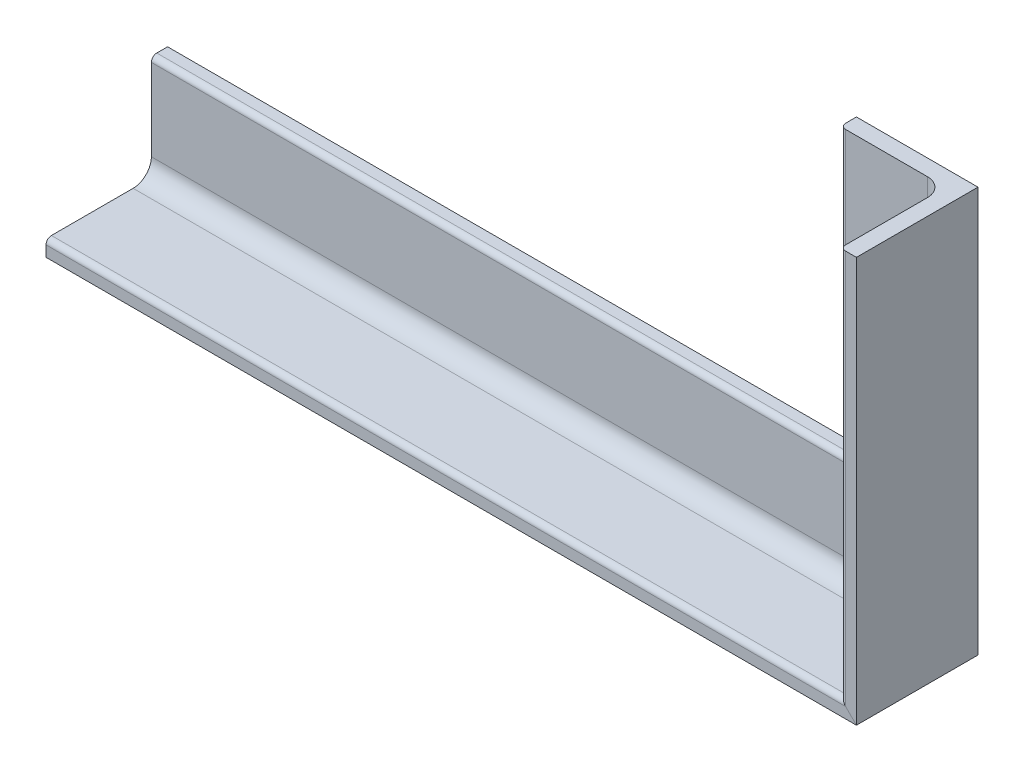
SolidWorks part; units mm, degrees
ref_plane "前视基准面" through (0, 0, 0) normal (0, 0, 1) x (1, 0, 0)
ref_plane "上视基准面" through (0, 0, 0) normal (0, 1, 0) x (1, 0, 0)
ref_plane "右视基准面" through (0, 0, 0) normal (1, 0, 0) x (0, 0, -1)
sketch "草图1" plane through (0, 0, 0) normal (0, 0, 1) x (1, 0, 0)
  line L0 (0, 0) -> (200, 0)
  line L1 (55, 0) -> (-55, 0) construction
  line L2 (200, 0) -> (200, 100)
  dimension "D1" = 200
  dimension "D2" = 100
other "Gbt706-2008 热轧等边角钢 030×4(1)"
ref_plane "基准面1" through (0, 0, 0) normal (1, 0, 0) x (0, 1, 0)
sketch "Sketch12" plane through (0, 0, 0) normal (1, 0, 0) x (0, 1, 0)
  line L0 (0, 0) -> (0, 30)
  line L1 (0, 15) -> (4, 15) construction
  line L2 (4, 28.6667) -> (4, 8.5)
  line L3 (8.5, 4) -> (28.6667, 4)
  line L4 (15, 4) -> (15, 0) construction
  line L5 (30, 0) -> (0, 0)
  line L6 (0, 30) -> (2.6667, 30)
  line L7 (30, 0) -> (30, 2.6667)
  arc A0 (30, 2.6667) -> (28.6667, 4) centre (28.6667, 2.6667) ccw
  arc A1 (2.6667, 30) -> (4, 28.6667) centre (2.6667, 28.6667) cw
  arc A2 (8.5, 4) -> (4, 8.5) centre (8.5, 8.5) cw
  point P10 (15, 0)
  point P14 (0, 15)
  point P15 (4, 15)
  point P16 (15, 4)
  point P17 (4, 30)
  point P18 (30, 4)
  point P21 (30, 4)
  point P24 (4, 30)
  point P25 (0, 0)
equation "\"D2@Sketch12\" = \"D1@Sketch12\" / 3"
